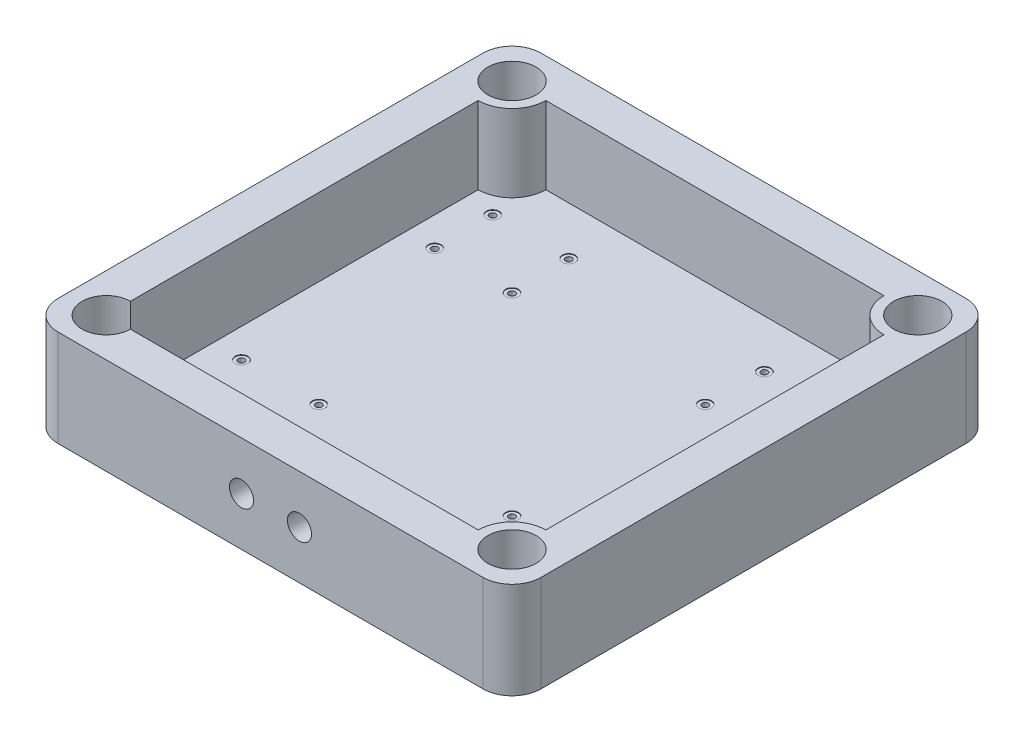
SolidWorks part; units mm, degrees
ref_plane "Front Plane" through (0, 0, 0) normal (0, 0, 1) x (1, 0, 0)
ref_plane "Top Plane" through (0, 0, 0) normal (0, 1, 0) x (1, 0, 0)
ref_plane "Right Plane" through (0, 0, 0) normal (1, 0, 0) x (0, 0, -1)
sketch "Sketch1" plane through (0, 0, 0) normal (0, 1, 0) x (1, 0, 0)
  line L1 (-220, -250) -> (220, -250)
  line L2 (-250, -220) -> (-250, 220)
  line L3 (-220, 250) -> (220, 250)
  line L4 (250, -220) -> (250, 220)
  line L5 (-250, -250) -> (250, 250) construction
  line L6 (-250, 250) -> (250, -250) construction
  arc A0 (-220, -250) -> (-250, -220) centre (-220, -220) cw
  arc A1 (-250, 220) -> (-220, 250) centre (-220, 220) cw
  arc A2 (250, 220) -> (220, 250) centre (220, 220) ccw
  arc A3 (220, -250) -> (250, -220) centre (220, -220) ccw
  point P0 (0, 0)
  dimension "D1" = 30
  dimension "D2" = 30
  dimension "D3" = 30
  dimension "D4" = 30
  dimension "D5" = 500
  dimension "D6" = 500
extrude "Boss-Extrude1" add sketch "Sketch1" along normal blind 100
sketch "Sketch2" plane through (0, 100, 0) normal (0, 1, 0) x (1, 0, 0)
  line L0 (0, 417.004) -> (0, -331.6209) construction
  line L5 (-175, -210) -> (175, -210)
  line L6 (-210, -175) -> (-210, 175)
  line L7 (-175, 210) -> (175, 210)
  line L8 (210, -175) -> (210, 175)
  line L9 (-210, -210) -> (210, 210) construction
  line L10 (-210, 210) -> (210, -210) construction
  line L11 (-372.8216, 0) -> (382.937, 0) construction
  line L12 (-210, 175) -> (210, 175) construction
  line L13 (175, 210) -> (175, -210) construction
  line L14 (210, -175) -> (-210, -175) construction
  line L15 (-175, 210) -> (-175, -210) construction
  arc A1 (175, 210) -> (210, 175) centre (210, 210) ccw
  arc A3 (-175, 210) -> (-210, 175) centre (-210, 210) cw
  arc A8 (175, -210) -> (210, -175) centre (210, -210) cw
  arc A9 (-175, -210) -> (-210, -175) centre (-210, -210) ccw
  point P0 (0, 0)
  dimension "D1" = 420
  dimension "D2" = 420
extrude "Cut-Extrude1" cut sketch "Sketch2" against normal blind 80
sketch "Sketch3" plane through (0, 100, 0) normal (0, 1, 0) x (1, 0, 0)
  line L0 (-471.3549, 0) -> (455.5106, 0) construction
  line L1 (0, 559.6412) -> (0, -544.8116) construction
  circle A0 centre (-210, 210) radius 25
  circle A2 centre (210, 210) radius 25
  circle A3 centre (210, -210) radius 25
  circle A4 centre (-210, -210) radius 25
  dimension "D1" = 210
  dimension "D2" = 210
extrude "Cut-Extrude2" cut sketch "Sketch3" against normal blind 80
sketch "Sketch4" plane through (0, 0, 0) normal (0, -1, 0) x (1, 0, 0)
  line L0 (-355.5467, 0) -> (494.8667, 0) construction
  line L5 (0, 399.4731) -> (0, -445.848) construction
  circle A1 centre (-150, -150) radius 20
  circle A2 centre (150, -150) radius 20
  circle A3 centre (150, 150) radius 20
  circle A4 centre (-150, 150) radius 20
  dimension "D1" = 150
  dimension "D2" = 150
sketch "Sketch10" plane through (0, 0, 250) normal (0, 0, 1) x (1, 0, 0)
  line L0 (0, 0) -> (0, 100) construction
  line L1 (-220, 100) -> (220, 100) construction
  line L2 (-220, 50) -> (220, 50) construction
  line L3 (-220, 100) -> (-220, 0) construction
  line L4 (220, 100) -> (220, 0) construction
  circle A0 centre (-30, 50) radius 12.5
  circle A1 centre (30, 50) radius 12.5
  point P15 (0, 50)
  dimension "D1" = 25
  dimension "D2" = 25
  dimension "D3" = 30
  dimension "D4" = 30
extrude "Cut-Extrude4" cut sketch "Sketch10" against normal blind 40
hole_wizard "CBORE for M6 Hexagon head bolts-Full thread-grade C1" positions "3DSketch2" profile "Sketch12" counterbore size "M6" standard "GB" end condition through all
sketch3d "3DSketch2"
  line L0 (-210, 20, -175) -> (-210, 20, 175) construction
  line L2 (-175, 20, 210) -> (175, 20, 210) construction
  point P0 (-180, 20, 100)
  point P2 (-100, 20, 100.0133)
  point P4 (-180, 20, 160)
  point P6 (-101.2651, 20, 160)
  dimension "D1" = 80
  dimension "D2" = 60
  dimension "D3" = 60
  dimension "D4" = 30
  dimension "D6" = 50
  dimension "D5" = 30
  dimension "D7" = 50
sketch "Sketch12" plane through (-180, 20, 100) normal (1, 0, 0) x (0, 0, 1)
  line L0 (0, 0) -> (0, 20)
  line L1 (0, 20) -> (3.3, 20)
  line L3 (3.3, 20) -> (3.3, 0.5)
  line L4 (6.5, 0.5) -> (3.3, 0.5)
  line L5 (6.5, 0.5) -> (6.5, 0.025)
  line L6 (6.5, 0.025) -> (6.525, 0)
  line L7 (6.525, 0) -> (0, 0)
  line L8 (-6.5, 0.025) -> (-6.525, 0) construction
  line L11 (0, -6.35) -> (0, 107.95) construction
  dimension "通孔孔直径" = 6.6
  dimension "通孔孔深度" = 20
  dimension "柱形沉头孔直径" = 13
  dimension "柱形沉头孔深度" = 0.5
  dimension "近端锥形沉头孔直径" = 13.05
  dimension "近端锥形沉头孔角度" = 90
sketch "Sketch13" plane through (0, 20, 0) normal (0, 1, 0) x (1, 0, 0)
  line L0 (0, 250) -> (0, -250) construction
  line L1 (220, 250) -> (-220, 250) construction
  line L2 (-220, -250) -> (220, -250) construction
  line L3 (-210, 0) -> (250, 0) construction
  line L4 (-210, 175) -> (-210, -175) construction
  line L5 (250, -220) -> (250, 220) construction
ref_plane "Plane1" through (0, 0, 0) normal (1, 0, 0) x (0, 0, -1)
ref_plane "Plane2" through (0, 0, 0) normal (0, 0, 1) x (1, 0, 0)
mirror "Mirror1" about plane through (0, 0, 0) normal (0, 0, 1) of "CBORE for M6 Hexagon head bolts-Full thread-grade C1" second plane through (0, 0, 0) second plane normal (1, 0, 0)
sketch "Sketch14" plane through (0, 100, 0) normal (0, 1, 0) x (1, 0, 0)
  line L0 (-210, -175) -> (-210, -210)
  line L1 (-175, -210) -> (-210, -210)
  arc A0 (-210, -175) -> (-175, -210) centre (-210, -210) cw
extrude "Cut-Extrude5" cut sketch "Sketch14" against normal blind 80
equation "\"40、\"=10"
